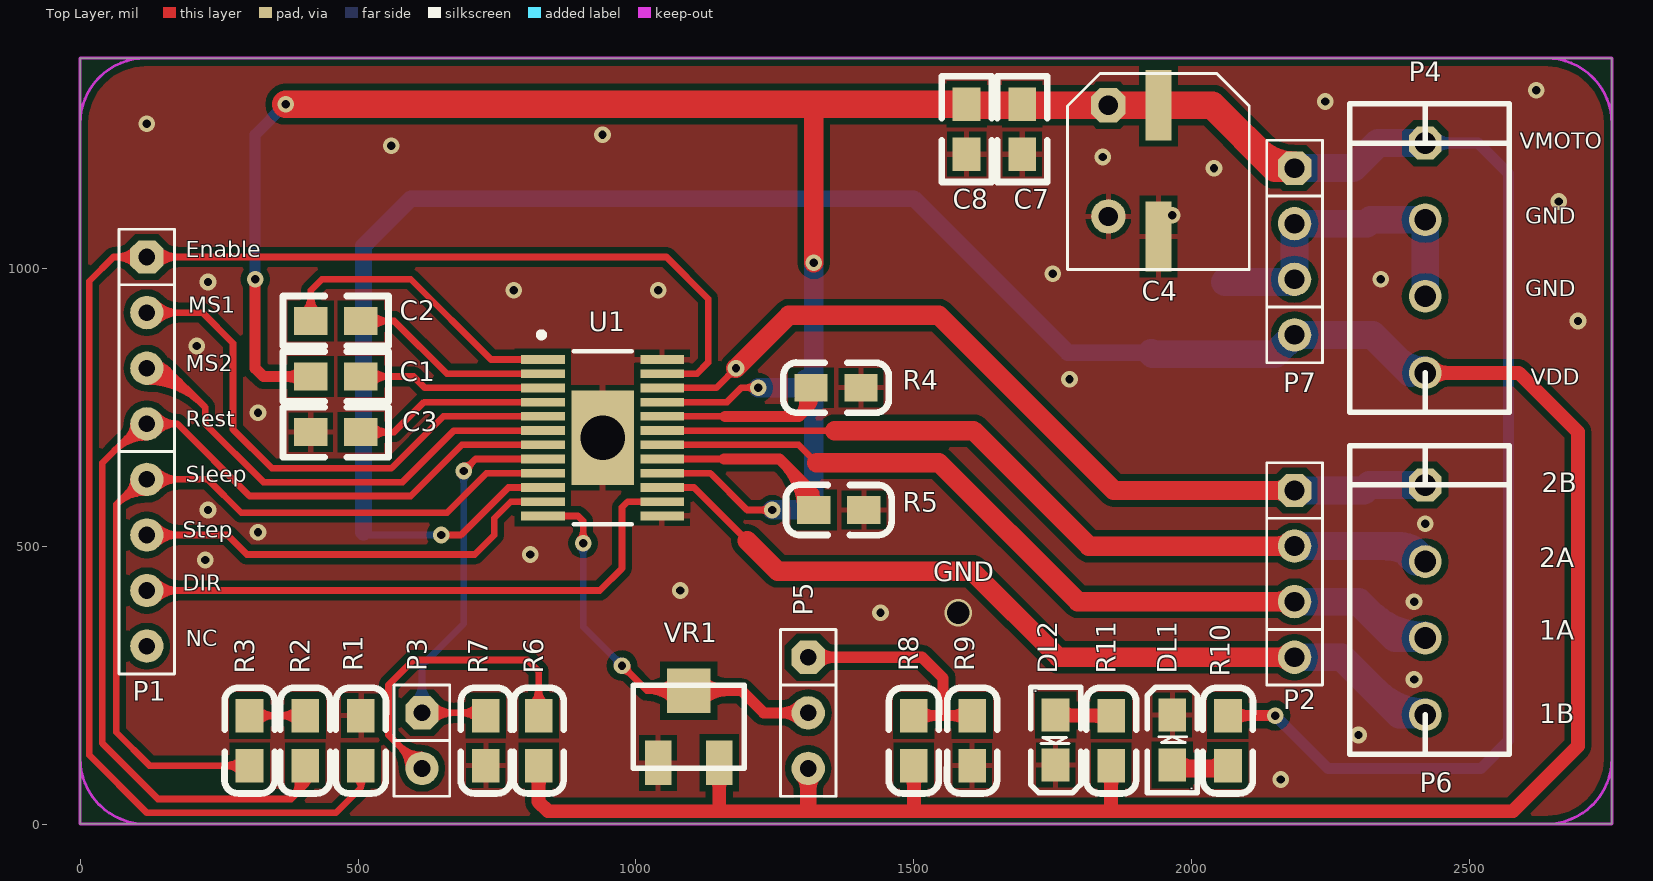
[diagram p0: Top Layer view]
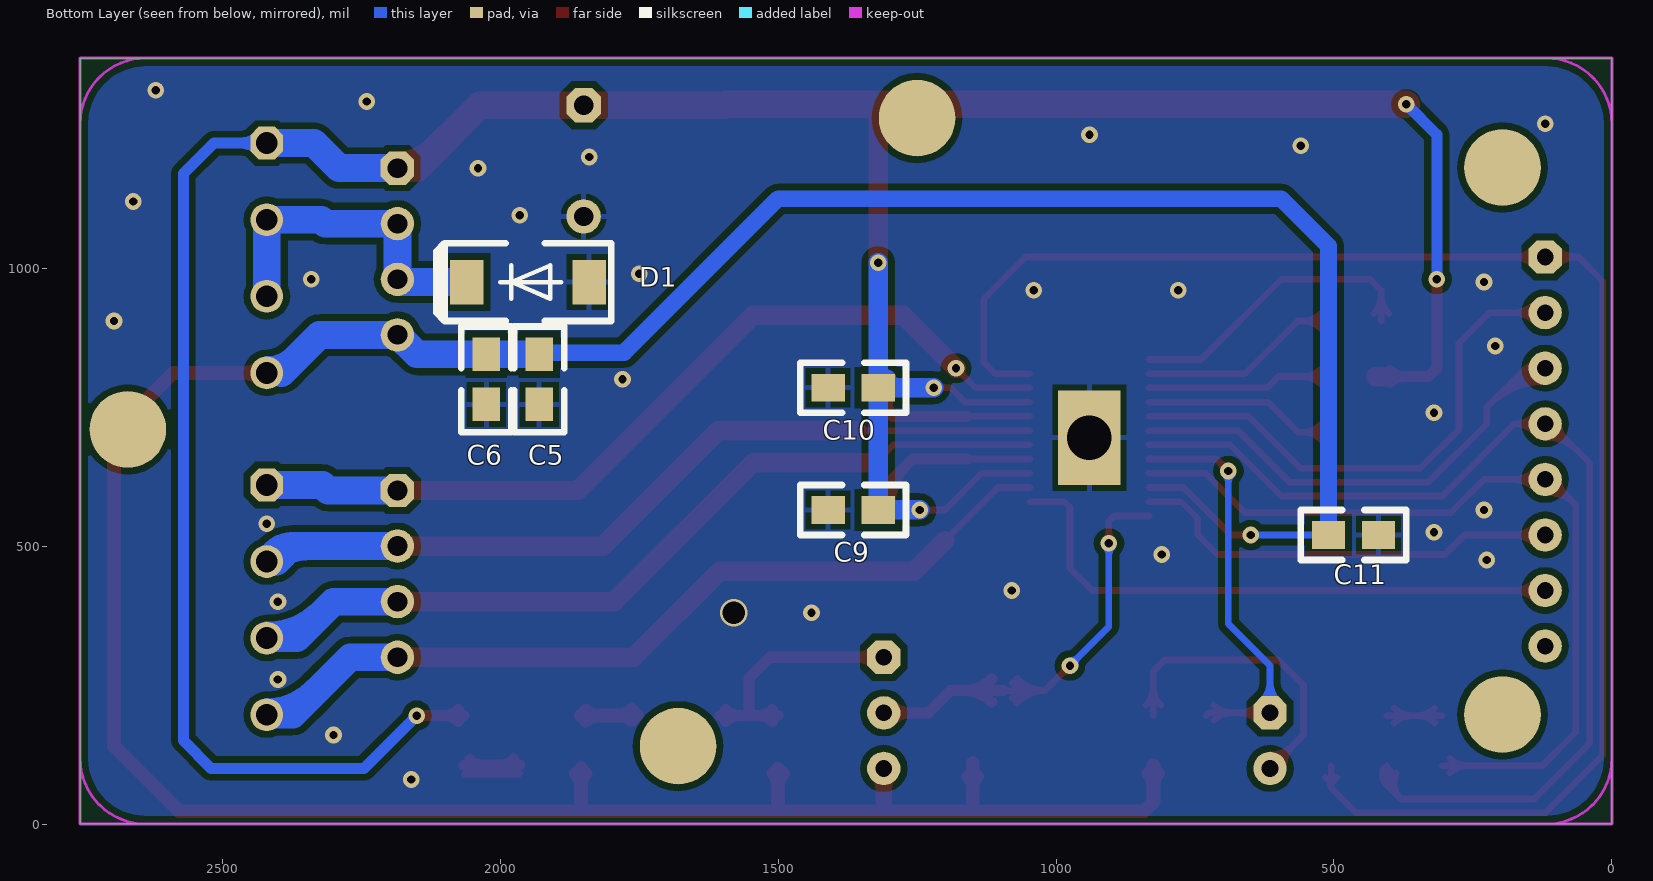
[diagram p1: Bottom Layer view, seen from below]
# Altium PCB MISC84410.PcbDoc
Units mil, origin at the board's own origin, x right, y up, seen from the top; angles counter-clockwise.
Board outline 2755.91 x 1377.95 mil, 2 copper layers (Top Layer, Bottom Layer); 34 components, 28 nets, 115 pads, 42 vias.

## Layer stack, top to bottom (the 12.6 mil dielectric is the usual default, probably not edited)
Top Solder: solder mask 0.4, Solder Resist, Dk 3.5
Top Layer: signal copper 1.4
Dielectric 1: dielectric 12.6, FR-4, Dk 4.8
Bottom Layer: signal copper 1.4
Bottom Solder: solder mask 0.4, Solder Resist, Dk 3.5

## Board outline
0,0 0,1377.95 2755.91,1377.95 2755.91,0

## Design rules (kind name [scope] priority, off if disabled: settings)
Clearance Ploy [InPolygon] p1: gap=12
Clearance [All] p2: gap=8
HoleSize [All] p1: absolutevalues=TRUE maxlimit=200 minlimit=1 maxpercent=80.000 minpercent=20.000
HoleToHoleClearance [All] p1: gap=5 allowstackedmicrovias=TRUE
MinimumSolderMaskSliver [All] p1: minsoldermaskwidth=0
PolygonConnect IsPloy [IsVia] p1: connectstyle=Direct reliefconductorwidth=10 reliefentries=4 polygonreliefangle="90 Angle" airgapwidth=10
PolygonConnect [All] p2: connectstyle=Relief reliefconductorwidth=10 reliefentries=4 polygonreliefangle="90 Angle" airgapwidth=10
RoutingVias [All] p1: holewidth=28 width=50 viastyle="Through Hole" minholewidth=12 minwidth=25 maxholewidth=100 maxwidth=100
SilkToBoardRegionClearance [All] p1 off:
SilkToSilkClearance [All] p1: silktosilkclearance=5
SilkToSolderMaskClearance [IsPad] p1: minsilkscreentomaskgap=0 clearancetoexposedcopper=TRUE
SolderMaskExpansion [All] p1: expansion=4
Width [All] p1: maxlimit=100 minlimit=8 preferedwidth=20
23 further rules are at their usual default settings.

## Components (designator, comment, footprint, x,y, rotation, side; value= is the part's Value field where it differs from the comment)
C1 "0.1uF" 0805C 460,805 r0 top
C2 "0.1uF" 0805C 460,905 r180 top
C3 "0.22uF" 0805C 460,705 r180 top
C4 "470uF" "CAP-SMD Aluminum Capacitors F8 220uF 35V" 1940,1175 r270 top
C5 "1uF" 0805C 1930,800 r270 bottom
C6 "0.1uF" 0805C 2025,800 r270 bottom
C7 "1uF" 0805C 1695,1250 r270 top
C8 "0.1uF" 0805C 1595,1250 r270 top
C9 "0.1uF" 0805C 1365,565 r0 bottom
C10 "0.1uF" 0805C 1365,785 r0 bottom
C11 "0.1uF" 0805C 465,520 r180 bottom
D1 "1N5822" 1N5822 1950,975 r0 bottom
DL1 "COLOR" 0805D 1965,151.05 r90 top
DL2 "COLOR" 0805D 1755,151.05 r270 top
P1 "Header(8PIN)" 排针（8PIN） 130,860 r270 top
P2 "Header(4PIN)" 排针(4PIN) 2185,500 r270 top
P3 "Header2PIN" 排针2PIN 615,150 r270 top
P4 "VH-3.5-4PIN" VH-3.5-4PIN 2420,1225 r270 top
P5 "Pin header (3PIN)" 排针(3PIN) 1310,300 r270 top
P6 "VH-3.5-4PIN" VH-3.5-4PIN 2420,610 r270 top
P7 "Header(4PIN)" 排针(4PIN) 2185,1080 r270 top
R1 "10KΩ" 0805R 505,150 r90 top
R2 "100KΩ" 0805R 405,150 r90 top
R3 "100KΩ" 0805R 305,150 r90 top
R4 "0.47Ω" 0805R 1360,785 r180 top
R5 "0.47Ω" 0805R 1365,565 r180 top
R6 "0Ω" 0805R 825,150 r270 top
R7 "0Ω" 0805R 730,150 r90 top
R8 "2KΩ" 0805R 1500,150 r90 top
R9 "3KΩ" 0805R 1605,150 r270 top
R10 "2.5KΩ" 0805R 2065,150 r270 top
R11 "4.7KΩ" 0805R 1855,150 r90 top
U1 "Value" A4982 940,695 r0 top
VR1 "10KΩ" 3224W 995,100 r0 top

## Footprints (in the part's own frame and the unit in brackets; to place one, negate y for a bottom-side part, rotate by r counter-clockwise, add the part's x,y. Pads: shape width x height; smd on the part's side, far side on the other; paste and mask are expansions set on the pad)
1N5822 [mil] "1N5822(3A/SMA)"
  rect 60x80 smd: 1(-110,0) 2(110,0)
  silkscreen extent -150,-70 165,70, body extent -108,-55 108,55, height 90
0805C [mil] "0805表贴电容"
  rect 60x50 smd: 1(-45,0) 2(45,0)
  silkscreen extent -95,-45 95,45, body extent -39,-23 39,24, height 37
0805D [mil] "表贴LED"
  rect 60x50 smd: 1(-45,0) 2(45,0)
  silkscreen extent -95,-45 95,45, body extent -41,-18 41,18, height 33
0805R [mil] "0805表贴电阻"
  rect 60x50 smd: 1(-45,0) 2(45,0)
  silkscreen extent -95,-45 95,45, body extent -39,-24 39,25, height 31
3224W [mil] "表贴电位器"
  rect 47.24x80 smd: 1(45,10) 3(155,10)
  rect 78.74x80 smd: 2(100,140)
  silkscreen extent 0,0 200,150, body extent 5,-15 195,180, height 146
A4982 [mm] "A4982"
  rect 2x0.4 smd: 1(-2.725,3.575) 2(-2.725,2.925) 3(-2.725,2.275) 4(-2.725,1.625) 5(-2.725,0.975) 6(-2.725,0.325) 7(-2.725,-0.325) 8(-2.725,-0.975) 9(-2.725,-1.625) 10(-2.725,-2.275) 11(-2.725,-2.925) 12(-2.725,-3.575) 13(2.725,-3.575) 14(2.725,-2.925) 15(2.725,-2.275) 16(2.725,-1.625) 17(2.725,-0.975) 18(2.725,-0.325) 19(2.725,0.325) 20(2.725,0.975) 21(2.725,1.625) 22(2.725,2.275) 23(2.725,2.925) 24(2.725,3.575)
  rect 2.85x4.32 smd: 24(0,0)
  rect 2.85x4.32 smd far side: 24(0,0)
  silkscreen extent -2.92,-3.95 1.32,4.83, body extent -2.25,-3.95 2.25,3.95, height 1.2
"CAP-SMD Aluminum Capacitors F8 220uF 35V" [mm] "SMD Aluminum Capacitors F8 220uF 35V"
  rect 3.2x1.2 smd: 1(-3,0) 2(3,0)
  silkscreen extent -4.45,-4.15 4.5,4.15, body extent -4.5,-4.15 4.5,4.15, height 11.9
VH-3.5-4PIN [mm] "VH-3.5-4PIN"
  oct 1.5x1.5 hole 1: 1(0,0)
  round 1.5 hole 1: 2(3.5,0) 3(7,0) 4(10.5,0)
  silkscreen extent -1.8,-3.45 12.3,3.85
排针2PIN [mil] "排针2PIN"
  oct 60x60 hole 30: 1(-50,0)
  round 60 hole 30: 2(50,0)
  silkscreen extent -100,-50 100,50, body extent -100,-50 100,50, height 398
排针(3PIN) [mil] "2.54排针"
  oct 60x60 hole 30: 1(0,0)
  round 60 hole 30: 2(100,0) 3(200,0)
  silkscreen extent -50,-50 250,50, body extent -50,-50 250,50, height 374
排针(4PIN) [mil] "2.54排针"
  oct 60x60 hole 35.43: 1(-100,0)
  round 60 hole 35.43: 2(0,0) 3(100,0) 4(200,0)
  silkscreen extent -150,-50 250,50, body extent -150,-50 250,50, height 374
排针（8PIN） [mil] "排针（8PIN）"
  oct 60x60 hole 30: 1(-160,-10)
  round 60 hole 30: 2(-60,-10) 3(40,-10) 4(140,-10) 5(240,-10) 6(340,-10) 7(440,-10) 8(540,-10)
  silkscreen extent -210,-60 590,40, body extent -210,-60 590,40, height 374

## Part data
C1 C2 C3 C5 C6 C7 C8 C9 C10 C11: library part CAP0805, "0805 SMD capacitor"
C4: library part CAP-AEC, "THT capacitor"
D1: library part IN5822
DL1 DL2: library part LED_0805, "LED_0805"
P1: library part "Header 8", "Header, 8-Pin"
P2 P4 P6 P7: library part "Header 4", "Header, 4-Pin"
P3: library part "Header 2", "Header, 2-Pin"
P5: library part "Header 3"
R1 R2 R3 R4 R5 R6 R7 R8 R9 R10 R11: library part RES0805, "0805 SMD resistor"
U1: library part A4982, "A4982"
VR1: library part RPOT, "RPOT-SMD-10KΩ"

## Free pads (board coordinates)
  round 137.8 smd far side: 0(196.85,196.85) 0(196.85,1181.1) 0(1250,1270) 0(1680,140) 0(2670,710)
  oct 62x62 hole 35: 1(1850,1293)
  round 62 hole 35: 2(1850,1093)

## Via types
v1: diameter 30, hole 15, Top Layer to Bottom Layer, tented both sides, 40 vias
v2: diameter 100, hole 80, Top Layer to Bottom Layer, 1 vias
v3: diameter 50, hole 40, Top Layer to Bottom Layer, 1 vias

## Nets (pads, with @x,y where several pads share a name; then routed paths per layer and width w, separated by ;. In a path a pad name is that pad's centre, name@x,y a point inside that pad or via, vN(x,y) a via of type N, cw(c..) or ccw(c..) an arc to the next point about the centre after c; other vN are vias at no path point)
1A: P2.3 P6.3 U1.18 | length 1675.9
  Top Layer w12: U1.18 1292.8,682.2 1325,650
  Top Layer w35: 1325,650 1545,650 1795,400 P2.3 ; P2.3@2176.16,391.16 ccw(c2154.82,369.82) 2154.82,400 ccw(c2154.82,430.18) P2.3@2176.16,408.84
  Bottom Layer w50: P2.3 2300,400 2365.59,334.41 P6.3 ; 2319.39,380.61 ccw(c2420,481.22) P6.3@2420,338.94
1B: P2.4 P6.4 U1.15 | length 1686.4
  Top Layer w12: U1.15 1104.57,605.43 1200,510
  Top Layer w35: 1200,510 1255,455 1605,455 1760,300 P2.4 ; P2.4@2176.16,291.16 ccw(c2154.82,269.82) 2154.82,300 ccw(c2154.82,330.18) P2.4@2176.16,308.84
  Bottom Layer w50: P2.4 2270,300 2373.39,196.61 P6.4 ; 2332.7,237.3 ccw(c2420,324.61) P6.4@2420,201.14
2A: P2.2 P6.2 U1.19 | length 1695.5
  Top Layer w12: U1.19 1357.8,707.8
  Top Layer w35: 1357.8,707.8 1607.2,707.8 1815,500 P2.2 ; P2.2@2176.16,491.16 ccw(c2154.82,469.82) 2154.82,500 ccw(c2154.82,530.18) P2.2@2176.16,508.84
  Bottom Layer w50: P2.2 2375,500 ; 2341.97,500 cw(c2341.97,394.17) P6.2@2416.8,469 ; 2382.9,492.1 ccw(c2420,529.2) P6.2@2420,476.73 ; P6.2@2415.71,470.76 ccw(c2375,457.04) 2375,500 ; P6.2 2402.8,472.2 2375,500
2B: P2.1 P6.1 U1.22 | length 1642.9
  Top Layer w12: U1.22 1144.57,784.57 v1(1180,820) ; v1@1171,820 cw(c1149.27,820) 1164.64,804.64 cw(c1180,789.27) v1@1180,811
  Top Layer w35: v1(1180,820) 1275,915 1545,915 1860,600 P2.1 ; P2.1@2176.16,591.16 ccw(c2154.82,569.82) 2154.82,600 ccw(c2154.82,630.18) P2.1@2176.16,608.84
  Bottom Layer w50: P2.1 2310,600 2320,610 P6.1
GND: C3.2 C4.2 C5.2 C6.2 C7.2 C8.2 C9.2 C10.2 C11.2 D1.1 DL1.2 DL2.2 pad.2 R1.2 R4.1 R5.1 R7.1 R9.2 U1.13 U1.24 VR1.1
  other v1: 2160,80 2300,160 2400,260 1440,380 2400,400 1080,420 225,475 810,485 320,525 2420,540 230,565 320,740 1780,800 210,860 2695,905 780,960 1040,960 230,975 2340,980 1750,990 1965,1095 2660,1120 2040,1180 1840,1200 560,1220 940,1240 120,1260 2240,1300 2620,1320
  other v2: 940,695
  other v3: 1580,380
GND_M_C: D1.2 P4.2 P4.3 P7.2 P7.3 | length 605.8
  Bottom Layer w50: D1.2 2185,975 P7.3 P7.2 2315,1080 2322.2,1087.2 P4.2 P4.3
NetC1_2: C1.2 U1.3 | length 398.2
  Top Layer w12: C1.2@515,805 600,805 620.43,784.57 U1.3 ; C1.2@523.44,791.56 cw(c555.87,759.13) 555.87,805 cw(c555.87,850.87) C1.2@523.44,818.44
NetC2_1: C2.1 U1.2 | length 429.1
  Top Layer w12: C2.1@515,905 565,905 659.84,810.16 U1.2 ; C2.1@523.44,891.56 cw(c555.87,859.13) 555.87,905 cw(c555.87,950.87) C2.1@523.44,918.44
NetC2_2: C2.2 U1.1 | length 612.8
  Top Layer w12: C2.2@401.56,918.44 ccw(c369.13,950.87) 415,950.87 ccw(c460.87,950.87) C2.2@428.44,918.44 ; C2.2 415,960 435,980 595,980 739.25,835.75 U1.1
NetC3_1: C3.1 U1.4 | length 412.1
  Top Layer w12: C3.1@515,705 565,705 618.98,758.98 U1.4 ; C3.1@523.44,691.56 cw(c555.87,659.13) 555.87,705 cw(c555.87,750.87) C3.1@523.44,718.44
NetDL1_1: DL1.1 R10.2 | length 526.1
  Top Layer w12: DL1.1@1965,91.05 1966.05,90 R10.2@2065,90 ; DL1.1@1969.95,106 ccw(c2008.57,144.61) 2008.57,90 ; DL1.1@1978.44,114.48 ccw(c2037.54,173.58) 2037.54,90 ; 1994.99,90 ccw(c1994.99,170.01) R10.2@2051.56,113.44 ; 2023.96,90 ccw(c2023.96,141.04) R10.2@2060.05,104.95
  Top Layer w20: DL1.1 2063.95,106.05 R10.2 ; DL1.1@1975.61,95.44 cw(c2001.21,69.83) 2001.21,106.05 cw(c2001.21,142.26) DL1.1@1975.61,116.65 ; 2026.26,106.05 cw(c2026.26,66.26) R10.2@2054.39,94.39 ; 2031.31,106.05 ccw(c2031.31,138.69) R10.2@2054.39,115.61
NetDL2_1: DL2.1 R11.2 | length 195.2
  Top Layer w25: DL2.1 1756.05,195 R11.2 ; DL2.1@1763.84,187.21 cw(c1782.65,168.39) 1782.65,195 ; DL2.1@1763.84,204.88 ccw(c1787.7,228.75) 1787.7,195 ; R11.2@1846.16,186.16 ccw(c1824.82,164.82) 1824.82,195 ccw(c1824.82,225.18) R11.2@1846.16,203.84
NetP1_1: P1.1 R1.1 U1.23 | length 3038.5
  Top Layer w12: P1.1@103.03,1003.03 ccw(c62.06,962.06) 62.06,1020 ccw(c62.06,1077.94) P1.1@103.03,1036.97 ; P1.1@136.97,1003.03 cw(c177.94,962.06) 177.94,1020 cw(c177.94,1077.94) P1.1@136.97,1036.97 ; R1.1@494.65,84.07 cw(c482.27,65) 505,65 ; R1.1 505,65 ; R1.1@515.35,84.07 ccw(c527.73,65) 505,65 ; U1.23 1110.16,810.16 1130,830 1130,945 1055,1020 110,1020 60,1020 16.5,976.5 16.5,123.91 120.41,20 460,20 505,65
NetP1_2: P1.2 U1.5 | length 1059.2
  Top Layer w12: P1.2@110,920 220,920 275,865 275,710 345,640 560,640 653.39,733.39 U1.5 ; P1.2@136.97,903.03 cw(c177.94,862.06) 177.94,920 cw(c177.94,977.94) P1.2@136.97,936.97
NetP1_3: P1.3 U1.6 | length 1207.1
  Top Layer w12: P1.3@110,820 155,820 ; P1.3@120,796 cw(c120,653.56) 220.72,754.28 ; P1.3@120,808 cw(c120,694.53) 200.23,774.77 ; P1.3 cw(c120,735.5) 179.75,795.25 ; P1.3@120,832 cw(c120,776.47) 159.26,815.74 ; P1.3@142.39,811.35 cw(c155,806.48) 155,820 ; P1.3@142.39,828.65 ccw(c155,833.52) 155,820 ; U1.6 672.8,707.8 580,615 330,615 225,720 225,750 155,820
NetP1_4: P1.4 R2.1 U1.7 | length 2249.1
  Top Layer w12: 61.96,671.96 cw(c120,613.92) P1.4@120,696 ; 82.44,692.44 cw(c120,654.89) P1.4@120,708 ; 86.1,696.1 ccw(c62.2,720) P1.4@96,720 ; P1.4@137.6,703.68 cw(c175,668.99) 175,720 ; P1.4@137.6,736.32 ccw(c175,771.01) 175,720 ; R2.1@387.9,91.73 cw(c351.09,73.92) 380,45 ; 391.94,56.94 ccw(c367.17,81.7) R2.1@398.7,96.95 ; R2.1@396.88,82.82 cw(c390.82,70) 405,70 ; 403.87,68.87 ccw(c383.26,89.48) R2.1@409.5,102.18 ; R2.1 405,70 ; R2.1@413.12,82.82 ccw(c419.18,70) 405,70 ; U1.7 687.2,682.2 595,590 305,590 175,720 ; 175,720 110,720 40,650 40,145 140,45 380,45 ; 380,45 405,70
NetP1_5: P1.5 R3.1 U1.9 | length 1810.6
  Top Layer w12: 84.31,594.31 cw(c117.49,561.14) P1.5@119.49,608.01 ; 86.1,596.1 ccw(c62.2,620) P1.5@96,620 ; P1.5@110,615 P1.5@115,620 ; P1.5@118.98,596.02 ccw(c115.91,524.1) 65,575 ; P1.5@136.97,603.03 cw(c177.94,562.06) 177.94,620 cw(c177.94,677.94) P1.5@136.97,636.97 ; R3.1@291.56,91.56 ccw(c259.13,59.13) 259.13,105 ccw(c259.13,150.87) R3.1@291.56,118.44 ; R3.1 125,105 65,165 65,575 ; U1.9 731.02,631.02 660,560 290,560 230,620 P1.5@115,620 ; 65,575 110,620 P1.5@115,620
NetP1_6: P1.6 U1.11 | length 885.1
  Top Layer w12: P1.6@110,520 P1.6 265,520 300,485 710,485 745,520 745,550 774.84,579.84 U1.11 ; P1.6@136.97,503.03 cw(c177.94,462.06) 177.94,520 cw(c177.94,577.94) P1.6@136.97,536.97
NetP1_7: P1.7 U1.14 | length 1158.9
  Top Layer w12: P1.7@110,420 P1.7 935,420 975,460 975,569.84 985,579.84 U1.14 ; P1.7@136.97,403.03 cw(c177.94,362.06) 177.94,420 cw(c177.94,477.94) P1.7@136.97,436.97
NetP3_1: P3.1 R7.2 U1.8 | length 1069.2
  Top Layer w12: P3.1@605,200 610,195 P3.1@615,195 ; P3.1 725,200 R7.2 ; P3.1@631.97,183.03 cw(c672.94,142.06) 672.94,200 cw(c672.94,257.94) P3.1@631.97,216.97 ; v1(690,635) 711.61,656.61 U1.8 ; v1@690,644 ccw(c690,665.73) 705.36,650.36 ccw(c720.73,635) v1@699,635 ; R7.2@716.56,186.56 ccw(c684.13,154.13) 684.13,200 ccw(c684.13,245.87) R7.2@716.56,213.44
  Bottom Layer w12: P3.1@598.03,216.97 ccw(c557.06,257.94) 615,257.94 ccw(c672.94,257.94) P3.1@631.97,216.97 ; P3.1 615,285 690,360 v1(690,635) ; v1@683.64,628.64 cw(c668.27,613.27) 690,613.27 cw(c711.73,613.27) v1@696.36,628.64
NetP3_2: P3.2 R6.1 | length 714.8
  Top Layer w12: P3.2@591,100 ccw(c533.06,100) 574.03,140.97 ccw(c615,181.94) P3.2@615,124 ; P3.2 555,160 555,250 600,295 805,295 825,275 R6.1 ; R6.1@811.56,213.44 ccw(c779.13,245.87) 825,245.87 ccw(c870.87,245.87) R6.1@838.44,213.44
NetP5_1: P5.1 R8.2 R9.1 | length 620.1
  Top Layer w20: P5.1 1515,300 1552.5,262.5 1552.5,195 ; P5.1@1324.14,285.86 cw(c1358.28,251.72) 1358.28,300 cw(c1358.28,348.28) P5.1@1324.14,314.14 ; R8.2 1552.5,195 ; R8.2@1510.61,184.39 cw(c1536.21,158.79) 1536.21,195 cw(c1536.21,231.21) R8.2@1510.61,205.61 ; R9.1@1594.39,184.39 ccw(c1568.79,158.79) 1568.79,195 ccw(c1568.79,231.21) R9.1@1594.39,205.61 ; R9.1 1552.5,195
NetP5_2: P5.2 U1.12 VR1.2 | length 1244.7
  Top Layer w12: U1.12 895.75,554.25 905,545 v1(905,505) ; v1@898.64,511.36 ccw(c883.27,526.73) 905,526.73 ccw(c926.73,526.73) v1@911.36,511.36 ; v1@975,276 cw(c975,254.27) 990.36,269.64 cw(c1005.73,285) v1@984,285 ; v1(975,285) 1020,240 ; VR1.2@1070.21,217.66 ccw(c1020,172.41) 1020,240 ; VR1.2@1070.21,262.34 cw(c1020,307.59) 1020,240 ; VR1.2@1079.13,225.69 ccw(c1046.97,196.72) 1046.97,240 ccw(c1046.97,283.28) VR1.2@1079.13,254.31 ; VR1.2 1020,240
  Top Layer w20: VR1.2 1190,240 1230,200 P5.2 ; VR1.2@1115.77,219.23 cw(c1165.91,169.09) 1165.91,240 cw(c1165.91,310.91) VR1.2@1115.77,260.77 ; P5.2@1295.86,185.86 ccw(c1261.72,151.72) 1261.72,200 ccw(c1261.72,248.28) P5.2@1295.86,214.14
  Bottom Layer w12: v1@898.64,498.64 cw(c883.27,483.27) 905,483.27 cw(c926.73,483.27) v1@911.36,498.64 ; v1(905,505) 905,355 v1(975,285) ; v1@966,285 ccw(c944.27,285) 959.64,300.36 ccw(c975,315.73) v1@975,294
NetR4_2: R4.2 U1.20 | length 436
  Top Layer w12: U1.20 1160,733.39
  Top Layer w20: 1160,733.39 1293.39,733.39 ; R4.2@1297.56,776.62 cw(c1269.24,757.54) 1293.39,733.39 ; R4.2@1306,773 cw(c1292.5,755) 1315,755 ; 1310.55,750.55 ccw(c1289.75,771.35) R4.2@1314.15,787.79 ; R4.2 1315,755 ; R4.2@1324,773 ccw(c1337.5,755) 1315,755 ; 1293.39,733.39 1315,755
NetR5_2: R5.2 U1.17 | length 521.7
  Top Layer w12: U1.17 1158.39,656.61
  Top Layer w20: 1158.39,656.61 1258.39,656.61 1320,595 ; 1264.64,650.36 cw(c1179.29,565) R5.2@1300,565 ; 1298.79,616.21 cw(c1247.57,565) R5.2 1320,595 ; R5.2@1311,577 ccw(c1297.5,595) 1320,595 ; R5.2@1329,577 cw(c1342.5,595) 1320,595
VCC: R2.2 R3.2 | length 244.1
  Top Layer w12: R3.2 R2.2 ; R3.2@318.44,181.56 cw(c350.87,149.13) 350.87,195 cw(c350.87,240.87) R3.2@318.44,208.44 ; R2.2@391.56,181.56 ccw(c359.13,149.13) 359.13,195 ccw(c359.13,240.87) R2.2@391.56,208.44
VDD: C5.1 C6.1 C11.1 P4.4 P5.3 P7.4 R6.2 R8.1 R11.1 U1.10 VR1.3 | length 6530.3
  Top Layer w12: v1(650,520) 685,520 770.43,605.43 U1.10
  Top Layer w25: R6.2@816.16,91.16 cw(c794.82,69.82) 825,69.82 cw(c855.18,69.82) R6.2@833.84,91.16 ; R6.2 825,40 842,23 1150,23 ; VR1.3@1142.14,85.76 cw(c1123.15,66.77) 1150,66.77 cw(c1176.85,66.77) VR1.3@1157.86,85.76 ; VR1.3 1150,23 ; R8.1@1491.16,91.16 cw(c1469.82,69.82) 1500,69.82 cw(c1530.18,69.82) R8.1@1508.84,91.16 ; R8.1@1500,98.95 1500,28 1495,23 ; R11.1@1846.16,91.16 cw(c1824.82,69.82) 1855,69.82 cw(c1885.18,69.82) R11.1@1863.84,91.16 ; R11.1@1855,100 1855,23 ; P4.4 2588.39,811.61 2695,705 2695,140 2578,23 1855,23 ; P4.4@2432.04,799.57 cw(c2461.11,770.51) 2461.11,811.61 cw(c2461.11,852.72) P4.4@2432.04,823.65 ; 1150,23 1495,23 ; 1495,23 1855,23
  Top Layer w30: P5.3@1299.39,89.39 cw(c1273.79,63.79) 1310,63.79 cw(c1346.21,63.79) P5.3@1320.61,89.39 ; 1310,30.5 P5.3
  Bottom Layer w12: C11.1@510,525 515,520 v1(650,520)
  Bottom Layer w30: C11.1@510,525 510,1040 595,1125 1500,1125 1777,848 C5.1@1927,848 ; P4.4@2393.39,811.61 P4.4
  Bottom Layer w50: C5.1@1927,848 C5.1 C6.1 2150,845 P7.4 2325,880 P4.4@2393.39,811.61 ; 2366.84,838.16 ccw(c2420,891.32) P4.4@2420,816.14
VMOTO: C1.1 C4.1 C7.1 C8.1 C9.1 C10.1 P4.1 P7.1 pad.1 R10.1 U1.16 U1.21 | length 6156.9
  Top Layer w12: U1.16 1133.98,631.02 1200,565 v1(1245,565) ; U1.21 1163.98,758.98 1190,785 v1(1220,785) ; v1@1213.64,778.64 ccw(c1198.27,763.27) 1198.27,785 ccw(c1198.27,806.73) v1@1213.64,791.36 ; v1@1238.64,558.64 ccw(c1223.27,543.27) 1223.27,565 ccw(c1223.27,586.73) v1@1238.64,571.36
  Top Layer w20: v1(315,980) 315,820 330,805 C1.1 ; C1.1@399.39,794.39 ccw(c373.79,768.79) 373.79,805 ccw(c373.79,841.21) C1.1@399.39,815.61 ; R10.1 v1(2150,195) ; R10.1@2075.61,184.39 cw(c2101.21,158.79) 2101.21,195 cw(c2101.21,231.21) R10.1@2075.61,205.61
  Top Layer w35: C1.1 C1.1@425,805 ; v1(1320,1010) 1320,1290 1325,1295
  Top Layer w50: v1(370,1295) 1325,1295 C8.1 1596.89,1293.11 C4.1 2036.89,1293.11 2150,1180 P7.1 ; 2116.72,1213.28 ccw(c2185,1281.57) P7.1@2185,1185
  Bottom Layer w20: v1(315,980) 315,1240 v1(370,1295) ; v1(2150,195) 2245,100 2520,100 2570,150 2570,1170 2515,1225 P4.1 ; P4.1@2433.81,1211.19 cw(c2467.14,1177.86) 2467.14,1225 cw(c2467.14,1272.14) P4.1@2433.81,1238.81
  Bottom Layer w35: v1(1220,785) C10.1 ; v1(1245,565) C9.1 C10.1 ; C10.1@1305,800 C10.1 ; v1(1320,1010) C10.1
  Bottom Layer w50: P7.1 2290,1180 2335,1225 P4.1
pads on no net: P1.8

## Polygon pours and split planes (outlines as drawn)
GND on Top Layer "Top Layer" (solid, remove dead copper, pour order 7): 0,1377.95 0,0 1005,0 2755.91,0 2755.91,795 2755.91,1377.95 0,1377.95
GND on Bottom Layer "Top Layer" (solid, remove dead copper, pour order 7): 0,1377.95 0,0 1005,0 2755.91,0 2755.91,795 2755.91,1377.95 0,1377.95

## Keep-outs
Keep-Out Layer:
  lines w5: 0,118.11 ccw(c118.11,118.11) 118.11,0 ; 0,1259.84 cw(c118.11,1259.84) 118.11,1377.95 ; 2637.8,0 ccw(c2637.8,118.11) 2755.91,118.11 ; 2637.8,1377.95 cw(c2637.8,1259.84) 2755.91,1259.84 ; 0,0 0,1377.95 2755.91,1377.95 2755.91,0 0,0

## Silkscreen, mask and mechanical layers (free items; w line width, h text height)
Top Overlay:
  text "VMOTO" at 2590,1205 h50
  text "GND" at 2600,1070 h50
  text "Enable" at 190,1010 h50
  text "GND" at 2600,940 h50
  text "MS1" at 195,910 h50
  text "MS2" at 190,805 h50
  text "VDD" at 2610,780 h50
  text "Rest" at 190,705 h50
  text "Sleep" at 190,605 h50
  text "2B" at 2630,585 h60
  text "Step" at 185,505 h50
  text "2A" at 2625,450 h60
  text "GND" at 1535,425 h60
  text "DIR" at 185,410 h50
  text "1A" at 2625,320 h60
  text "NC" at 190,310 h50
  text "1B" at 2625,170 h60
Mechanical 1:
  lines w5: -5000,-3380 -5000,4887.72 6692.91,4887.72 6692.91,-3380 -5000,-3380

## Dimensions
2755.91,1377.95 to 2755.91,0 on Keep-Out Layer
0,0 to 2755.91,0 on Keep-Out Layer